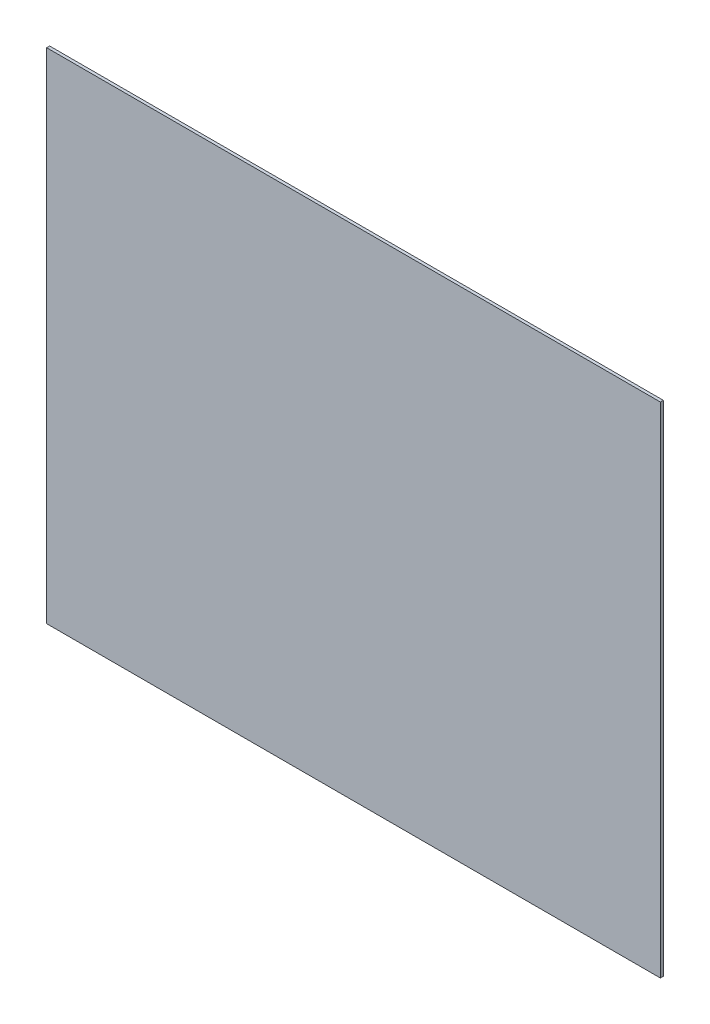
SolidWorks part; units mm, degrees
material "PMMA(有机玻璃)"
ref_plane "前视" through (0, 0, 0) normal (0, 0, 1) x (1, 0, 0)
ref_plane "上视" through (0, 0, 0) normal (0, 1, 0) x (1, 0, 0)
ref_plane "右视" through (0, 0, 0) normal (1, 0, 0) x (0, 0, -1)
sketch "草图1" plane through (0, 0, 0) normal (0, 0, 1) x (1, 0, 0)
  line L1 (-518.5, 421.5) -> (518.5, 421.5)
  line L2 (-518.5, 421.5) -> (-518.5, -421.5)
  line L3 (-518.5, -421.5) -> (518.5, -421.5)
  line L4 (518.5, 421.5) -> (518.5, -421.5)
  line L5 (-518.5, 421.5) -> (518.5, -421.5) construction
  line L6 (-518.5, -421.5) -> (518.5, 421.5) construction
  point P0 (0, 0)
  dimension "D1" = 843
  dimension "D2" = 1037
extrude "凸台-拉伸1" add sketch "草图1" along normal blind 5
hole_wizard "M5 间隙孔1" positions "草图3" profile "草图2" hole size "M5" standard "GB"
sketch "草图3" plane through (0, 0, 5) normal (0, 0, 1) x (1, 0, 0)
  line L0 (-427.5, 273) -> (-427.5, -273) construction
  line L1 (-427.5, -273) -> (427.5, -273) construction
  line L2 (0, 273) -> (0, -273) construction
  line L3 (427.5, 273) -> (-427.5, 273) construction
  line L5 (-427.5, 0) -> (427.5, 0) construction
  line L6 (427.5, -273) -> (427.5, 273) construction
  point P0 (-375, -261)
  point P46 (415.5, 250)
  point P48 (-415.5, 250)
  point P58 (-125, -261)
  point P59 (125, -261)
  point P61 (-125, 261)
  point P62 (125, 261)
  point P64 (-375, 261)
  point P88 (375, -261)
  point P89 (375, 261)
  point P108 (415.5, 0)
  point P109 (-415.5, 0)
  point P110 (415.5, -250)
  point P111 (-415.5, -250)
  dimension "D1" = 12
  dimension "D2" = 12
  dimension "D5" = 3
  dimension "D3" = 12
  dimension "D6" = 4
  dimension "D4" = 2
sketch "草图2" plane through (-375, -261, 5) normal (1, 0, 0) x (0, -1, 0)
  line L0 (0, 0) -> (0, 5)
  line L1 (0, 5) -> (2.75, 5)
  line L2 (2.75, 5) -> (2.75, 0)
  line L5 (2.75, 0) -> (0, 0)
  line L11 (0, -6.35) -> (0, 107.95) construction
  dimension "通孔孔直径" = 5.5
  dimension "通孔孔深度" = 5
